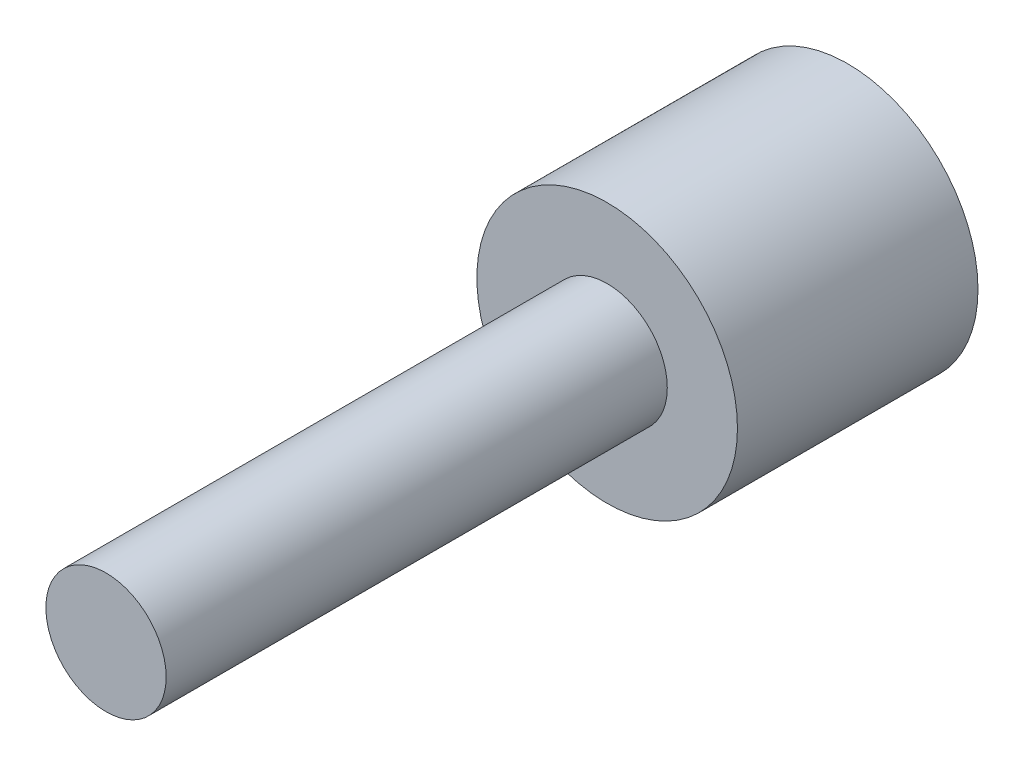
SolidWorks part; units mm, degrees
material "OTHER"
ref_plane "前视基准面" through (0, 0, 0) normal (0, 0, 1) x (1, 0, 0)
ref_plane "上视基准面" through (0, 0, 0) normal (0, 1, 0) x (1, 0, 0)
ref_plane "右视基准面" through (0, 0, 0) normal (1, 0, 0) x (0, 0, -1)
sketch "草图1" plane through (0, 0, 0) normal (0, 0, 1) x (1, 0, 0)
  circle A0 centre (0, 0) radius 6.5
  dimension "D1" = 13
extrude "凸台-拉伸1" add sketch "草图1" along normal blind 12
sketch "草图2" plane through (0, 0, 12) normal (0, 0, 1) x (1, 0, 0)
  circle A0 centre (0, 0) radius 3
  dimension "D1" = 6
extrude "凸台-拉伸2" add sketch "草图2" along normal blind 25
sketch "草图3" plane through (0, 0, 0) normal (0, 0, -1) x (-1, 0, 0)
  circle A0 centre (0, 0) radius 5
  dimension "D1" = 10
extrude "切除-拉伸1" cut sketch "草图3" against normal blind 0.5
